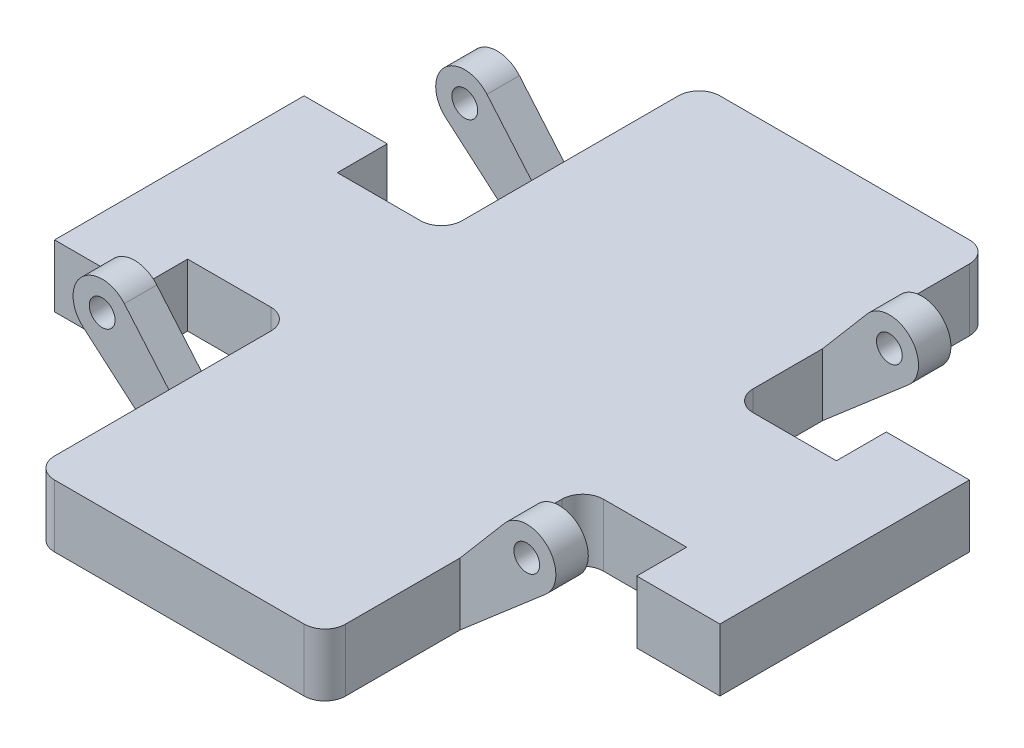
SolidWorks part; units mm, degrees
ref_plane "Front Plane" through (0, 0, 0) normal (0, 0, 1) x (1, 0, 0)
ref_plane "Top Plane" through (0, 0, 0) normal (0, 1, 0) x (1, 0, 0)
ref_plane "Right Plane" through (0, 0, 0) normal (1, 0, 0) x (0, 0, -1)
other "Configuration Table"
sketch "Sketch1" plane through (0, 0, 0) normal (0, 1, 0) x (1, 0, 0)
  line L1 (-65, -65) -> (65, -65)
  line L2 (-65, -65) -> (-65, 65)
  line L3 (-65, 65) -> (65, 65)
  line L4 (65, -65) -> (65, 65)
  line L5 (-65, -65) -> (65, 65) construction
  line L6 (-65, 65) -> (65, -65) construction
  point P0 (0, 0)
  dimension "D1" = 130
extrude "Boss-Extrude1" add sketch "Sketch1" along normal blind 15
sketch "Sketch2" plane through (0, 15, 0) normal (0, 1, 0) x (1, 0, 0)
  line L0 (-65, 65) -> (-35, 65)
  line L1 (65, 65) -> (-65, 65) construction
  line L2 (-35, 65) -> (-35, 20)
  line L3 (-35, 20) -> (35, 20)
  line L4 (0, 0) -> (0, 65) construction
  line L5 (35, 65) -> (35, 20)
  line L6 (65, 65) -> (35, 65)
  line L7 (20, 35) -> (20, -35)
  line L8 (65, -35) -> (20, -35)
  line L9 (65, 35) -> (20, 35)
  line L10 (35, -20) -> (-35, -20)
  line L11 (-35, -65) -> (-35, -20)
  line L12 (35, -65) -> (35, -20)
  line L13 (-20, -35) -> (-20, 35)
  line L14 (-65, 35) -> (-20, 35)
  line L15 (-65, -35) -> (-20, -35)
  line L16 (-65, -35) -> (-65, -65)
  line L17 (-65, -65) -> (65, -65)
  line L18 (65, -65) -> (65, 65)
  line L19 (-35, 65) -> (35, 65)
  line L20 (-65, 35) -> (-65, -35)
  line L21 (-65, 65) -> (-65, 35)
  circle A0 centre (0, 0) radius 13.6226 construction
  point P11 (0, 20)
  point P29 (0, 0)
  line M16 (65, -65) -> (65, 65)
  line M17 (65, 65) -> (-65, 65)
  line M18 (-65, 65) -> (-65, -65)
  line M19 (-65, -65) -> (65, -65)
  dimension "D2" = 4
  dimension "D1" = 30
extrude "Cut-Extrude1" cut sketch "Sketch2" against normal through all contours L15 L11 M18 M19 | L14 L2 M18 M17 | L9 L5 M16 M17 | L12 L8 M19 M16
sketch "Sketch5" plane through (0, 15, 0) normal (0, 1, 0) x (1, 0, 0)
  line L0 (-69.7955, 0) -> (70.4837, 0) construction
  line L1 (-48.5, 16.9588) -> (-48.5, -15.8857) construction
  line L3 (0, 75.4948) -> (0, -74.5052) construction
  circle A43 centre (0, 0) radius 48.5
  circle A44 centre (-48.5, 0) radius 7.5
  circle A45 centre (-48.5, 0) radius 12.5
  circle A46 centre (-38.5, 0) radius 1.5
  circle A47 centre (-58.5, 0) radius 1.5
  circle A48 centre (-48.5, 10) radius 1.5
  circle A49 centre (-48.5, -10) radius 1.5
  circle A50 centre (0, 0) radius 48.5
  circle A51 centre (10, 48.5) radius 1.5
  circle A52 centre (0, 38.5) radius 1.5
  circle A53 centre (-10, 48.5) radius 1.5
  circle A54 centre (0, 58.5) radius 1.5
  circle A55 centre (0, 0) radius 48.5
  circle A56 centre (48.5, -10) radius 1.5
  circle A57 centre (38.5, 0) radius 1.5
  circle A58 centre (48.5, 10) radius 1.5
  circle A59 centre (58.5, 0) radius 1.5
  circle A60 centre (0, 0) radius 48.5
  circle A61 centre (-10, -48.5) radius 1.5
  circle A62 centre (0, -38.5) radius 1.5
  circle A63 centre (10, -48.5) radius 1.5
  circle A64 centre (0, -58.5) radius 1.5
  point P49 (0, 0)
  dimension "D1" = 97
  dimension "D3" = 15
  dimension "D4" = 10
  dimension "D5" = 3
  dimension "D6" = 10
  dimension "D7" = 10
  dimension "D8" = 10
  dimension "D2" = 25
extrude "Cut-Extrude4" cut sketch "Sketch5" against normal through all from offset 10 contours A47 | A43 A49 | A60 A63 | A64 | A55 A56 | A55 A56 | A57 | A59 | A55 A58 | A55 A58 | A52 | A54 | A50 A51 | A50 A51 | A50 A53 | A50 A53 | A48 | A46 | A62 | A61 offset against normal yes
sketch "Sketch8" plane through (0, 15, 0) normal (0, 1, 0) x (1, 0, 0)
  line L0 (65, -35) -> (65, 35) construction
  line L1 (35, 35) -> (65, 35)
  line L2 (35, 35) -> (35, 18)
  line L3 (35, 18) -> (65, 18)
  line L4 (65, 35) -> (65, 18)
  line L5 (0, 0) -> (81.9164, 0) construction
  line L6 (0, 0) -> (0, 69.1421) construction
  line L7 (65, -35) -> (65, -18)
  line L8 (35, -18) -> (65, -18)
  line L9 (35, -35) -> (35, -18)
  line L10 (35, -35) -> (65, -35)
  line L11 (-65, 35) -> (-65, 18)
  line L12 (-35, 35) -> (-65, 35)
  line L13 (-35, -35) -> (-65, -35)
  line L14 (-35, -35) -> (-35, -18)
  line L15 (-35, -18) -> (-65, -18)
  line L16 (-65, -35) -> (-65, -18)
  line L17 (-35, 18) -> (-65, 18)
  line L18 (-35, 35) -> (-35, 18)
  dimension "D1" = 17
extrude "Cut-Extrude5" cut sketch "Sketch8" against normal through all
fillet "Fillet1" radius 5 12 edges at (-35, 7.5, 18) (-65, 7.5, 18) (-65, 7.5, -18) (-35, 7.5, -18) (-35, 7.5, -65) (35, 7.5, -65) (35, 7.5, -18) (65, 7.5, -18) (35, 7.5, 18) (65, 7.5, 18) (35, 7.5, 65) (-35, 7.5, 65)
sketch "Sketch9" plane through (0, 15, 0) normal (0, 1, 0) x (1, 0, 0)
  line L0 (35, 60) -> (35, 23) construction
  line L1 (-35, 60) -> (35, 60)
  line L2 (-35, 60) -> (-35, 80)
  line L3 (-35, 80) -> (35, 80)
  line L4 (35, 60) -> (35, 80)
  line L6 (35, -60) -> (35, -23) construction
  line L7 (-35, -60) -> (35, -60)
  line L8 (-35, -60) -> (-35, -80)
  line L9 (-35, -80) -> (35, -80)
  line L10 (35, -60) -> (35, -80)
  dimension "D1" = 20
  dimension "D2" = 20
extrude "Boss-Extrude3" add sketch "Sketch9" against normal blind 15
ref_plane "Plane1" through (0, 0, -43.6) normal (0, 0, -1) x (-1, 0, 0)
sketch "Sketch10" plane through (0, 0, -43.6) normal (0, 0, -1) x (-1, 0, 0)
  line L0 (35, 15) -> (45.7163, 27.6025)
  line L1 (55.6182, 17.7649) -> (35, 0)
  line L2 (35, 15) -> (35, 0)
  arc A0 (45.7163, 27.6025) -> (55.6182, 17.7649) centre (51.049, 23.068) cw
  circle A1 centre (51.049, 23.068) radius 3.1
  dimension "D1" = 7
  dimension "D2" = 6.2
extrude "Boss-Extrude4" add sketch "Sketch10" along normal mid plane 7.8
mirror "Mirror1" about plane through (0, 0, 0) normal (1, 0, 0) of "Boss-Extrude4"
mirror "Mirror2" about plane through (0, 0, 0) normal (0, 0, 1) of "Mirror1", "Boss-Extrude4"
fillet "Fillet2" radius 5 4 edges at (35, 7.5, 80) (-35, 7.5, 80) (35, 7.5, -80) (-35, 7.5, -80)
sketch "Sketch6" plane through (0, 0, 0) normal (1, 0, 0) x (0, 0, -1)
  line L0 (0, 47.8975) -> (0, -24.1044) construction
sketch "Sketch7" plane through (0, 15, 0) normal (0, 1, 0) x (1, 0, 0)
  line L1 (-30, 60) -> (30, 60)
  line L2 (-30, 60) -> (-30, 80)
  line L3 (-30, 80) -> (30, 80)
  line L4 (30, 60) -> (30, 80)
  line L5 (0, 0) -> (0, 60)
  line L6 (0, 0) -> (65, 0)
  line L7 (65, -13) -> (65, 13) construction
  line L8 (30, -60) -> (30, -80)
  line L9 (-30, -80) -> (30, -80)
  line L10 (-30, -60) -> (-30, -80)
  line L11 (-30, -60) -> (30, -60)
  line L13 (-60, 30) -> (-80, 30)
  line L14 (-60, 30) -> (-60, -30)
  line L15 (-60, -30) -> (-80, -30)
  line L16 (-80, 30) -> (-80, -30)
  line L17 (80, 30) -> (80, -30)
  line L18 (60, -30) -> (80, -30)
  line L19 (60, 30) -> (60, -30)
  line L20 (60, 30) -> (80, 30)
  dimension "D1" = 20
  dimension "D2" = 20
extrude "Boss-Extrude2" add sketch "Sketch7" along direction (0, -1, 0) on the side against the normal blind 15
